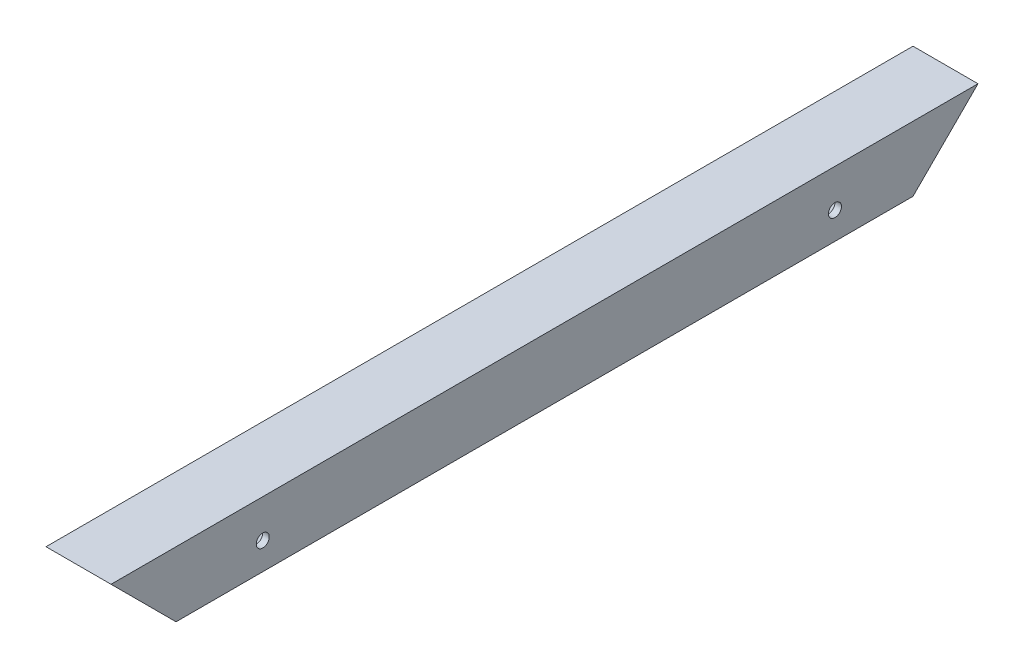
SolidWorks part; units mm, degrees
material "不锈钢管"
ref_plane "Front Plane" through (0, 0, 0) normal (0, 0, 1) x (1, 0, 0)
ref_plane "Top Plane" through (0, 0, 0) normal (0, 1, 0) x (1, 0, 0)
ref_plane "Right Plane" through (0, 0, 0) normal (1, 0, 0) x (0, 0, -1)
other "Configuration Table"
sketch "Sketch1" plane through (0, 0, 0) normal (0, 0, 1) x (1, 0, 0)
  line L0 (-45.1417, 25.901) -> (-15.1417, 25.901)
  line L1 (-15.1417, 25.901) -> (-15.1417, -4.099)
  line L2 (-15.1417, -4.099) -> (-45.1417, -4.099)
  line L3 (-45.1417, -4.099) -> (-45.1417, 25.901)
extrude "Boss-Extrude1" add sketch "Sketch1" along normal blind 400
sketch "Sketch2" plane through (0, 0, 400) normal (0, 0, 1) x (1, 0, 0)
  line L0 (-42.1417, 22.901) -> (-18.1417, 22.901)
  line L1 (-18.1417, 22.901) -> (-18.1417, -1.099)
  line L2 (-18.1417, -1.099) -> (-42.1417, -1.099)
  line L3 (-42.1417, -1.099) -> (-42.1417, 22.901)
  line L4 (-15.1417, -4.099) -> (-15.1417, 25.901) construction
  line L5 (-15.1417, 25.901) -> (-45.1417, 25.901) construction
  line L6 (-45.1417, 25.901) -> (-45.1417, -4.099) construction
  line L7 (-45.1417, -4.099) -> (-15.1417, -4.099) construction
  dimension "D1" = 3
  dimension "D2" = 3
  dimension "D3" = 3
  dimension "D4" = 3
extrude "Cut-Extrude1" cut sketch "Sketch2" against normal blind 492
sketch "Sketch4" plane through (-15.1417, 0, 0) normal (1, 0, 0) x (0, 0, -1)
  line L0 (0, 25.901) -> (-30, -4.099)
  line L1 (-400, -4.099) -> (0, -4.099) construction
  line L2 (-30, -4.099) -> (0, -4.099)
  line L3 (0, -4.099) -> (0, 25.901)
  dimension "D1" = 45
extrude "Cut-Extrude3" cut sketch "Sketch4" against normal through all
sketch "Sketch8" plane through (-15.1417, 0, 0) normal (1, 0, 0) x (0, 0, -1)
  line L0 (-400, 25.901) -> (-370, -4.099)
  line L1 (-400, -4.099) -> (-30, -4.099) construction
  line L2 (-370, -4.099) -> (-400, -4.099)
  line L3 (-400, -4.099) -> (-400, 25.901)
  dimension "D1" = 45
extrude "Cut-Extrude6" cut sketch "Sketch8" against normal through all
sketch "Sketch10" plane through (-15.1417, 0, 0) normal (1, 0, 0) x (0, 0, -1)
  line L0 (-450, 6.401) -> (-450, 12.401) construction
  line L1 (-453, 6.401) -> (-447, 6.401) construction
  line L2 (-447, 12.401) -> (-453, 12.401) construction
  line L3 (-456, 9.401) -> (-36, 9.401) construction
  line L4 (-42, 12.401) -> (-42, 6.401)
  line L5 (-39, 12.401) -> (-45, 12.401) construction
  line L6 (-45, 6.401) -> (-39, 6.401) construction
  line L7 (-306, 12.401) -> (-306, 6.401)
  line L8 (-303, 12.401) -> (-309, 12.401) construction
  line L9 (-309, 6.401) -> (-303, 6.401) construction
  line L10 (-186, 12.401) -> (-186, 6.401)
  line L11 (-183, 12.401) -> (-189, 12.401) construction
  line L12 (-189, 6.401) -> (-183, 6.401) construction
  arc A0 (-453, 12.401) -> (-453, 6.401) centre (-453, 9.401) ccw construction
  arc A1 (-39, 6.401) -> (-39, 12.401) centre (-39, 9.401) ccw construction
sketch "Sketch11" plane through (-15.1417, 0, 0) normal (1, 0, 0) x (0, 0, -1)
  line L0 (-370, -4.099) -> (-30, -4.099) construction
  circle A0 centre (-330, 8.401) radius 3
  circle A1 centre (-66, 8.401) radius 3
  dimension "D1" = 70
  dimension "D2" = 6
  dimension "D4" = 6
  dimension "D3" = 334
  dimension "D5" = 12.5
  dimension "D6" = 12.5
extrude "Cut-Extrude7" cut sketch "Sketch11" against normal through all both and the other way through all
